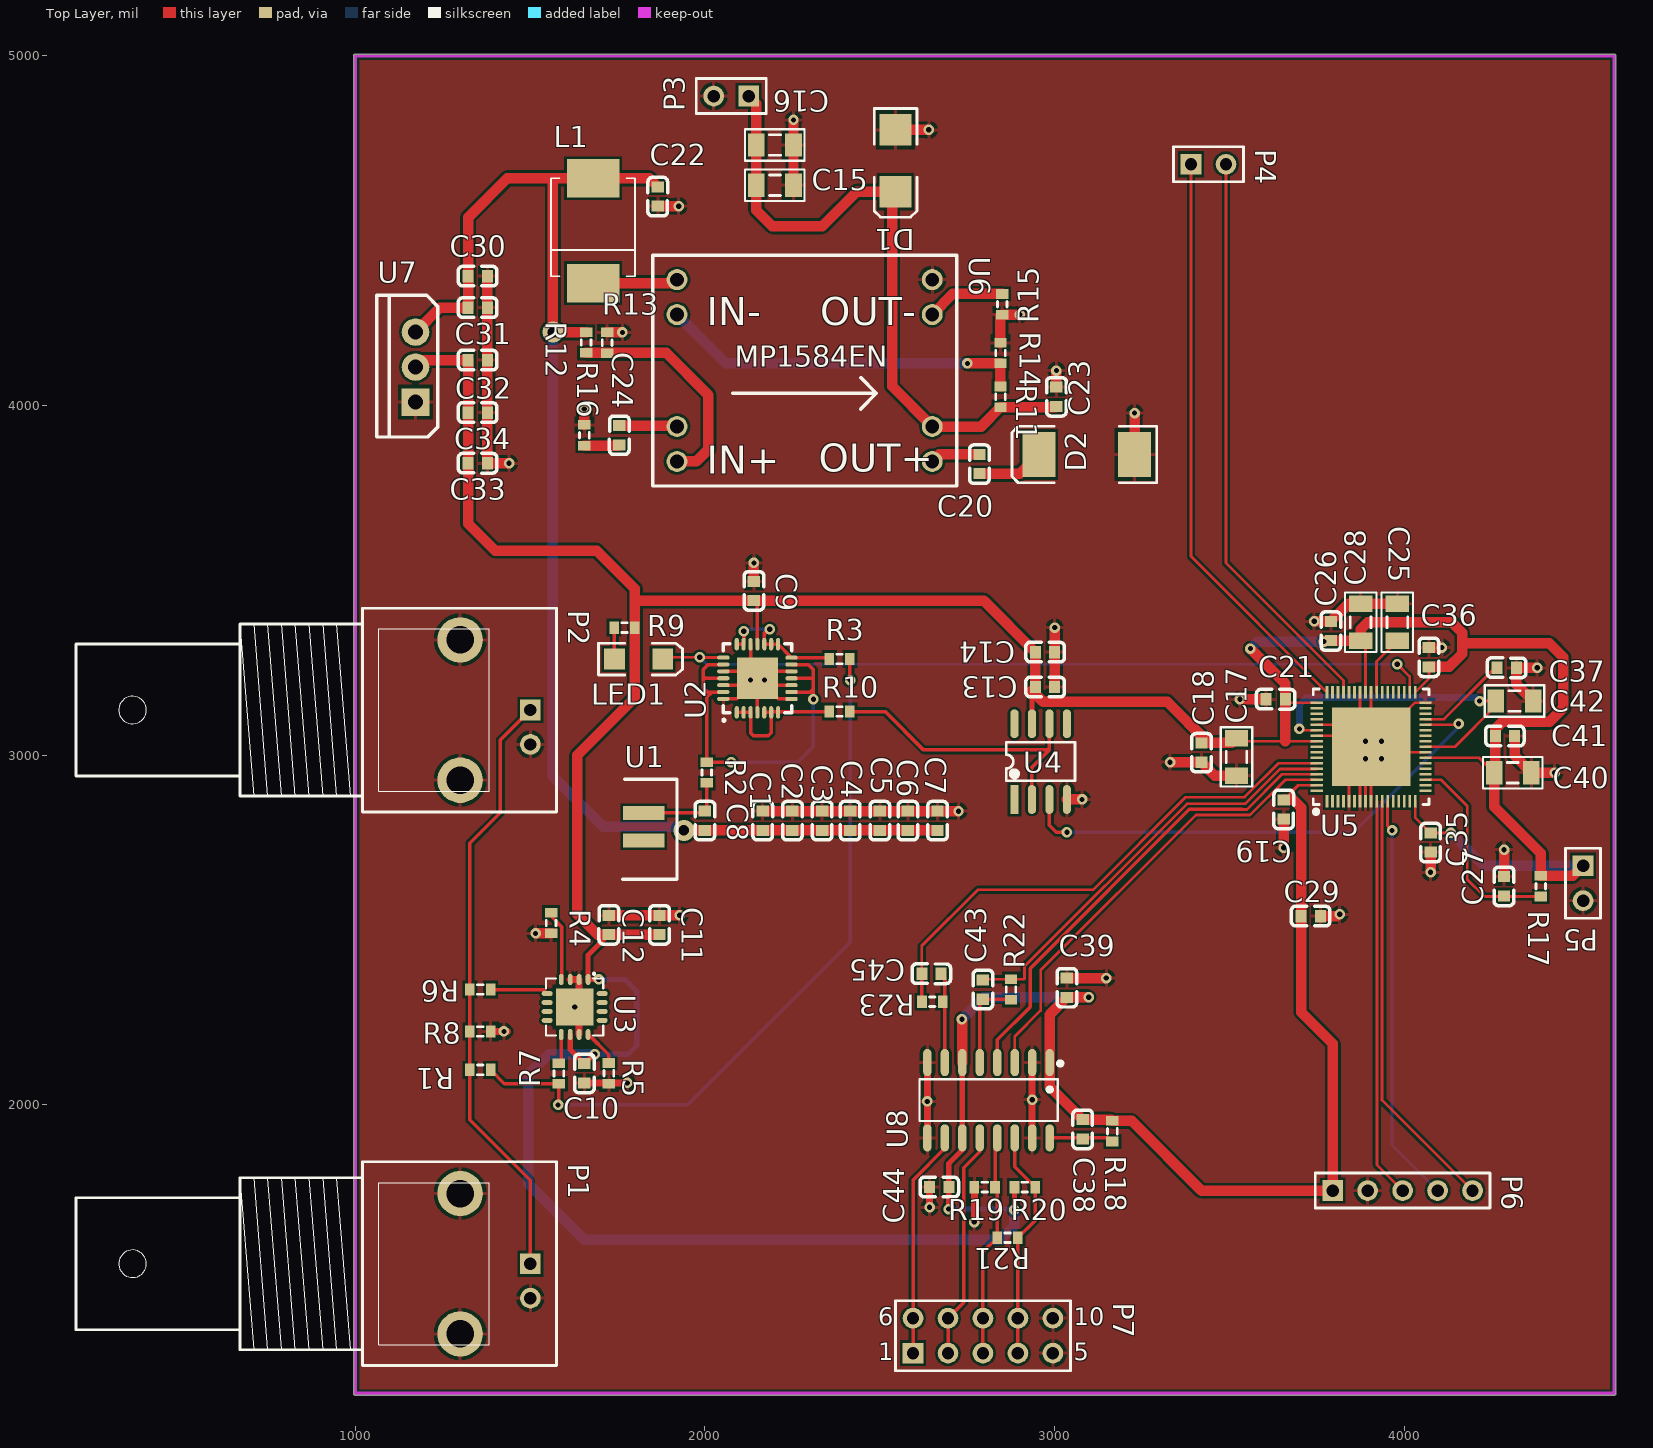
[diagram p0: Top Layer view]
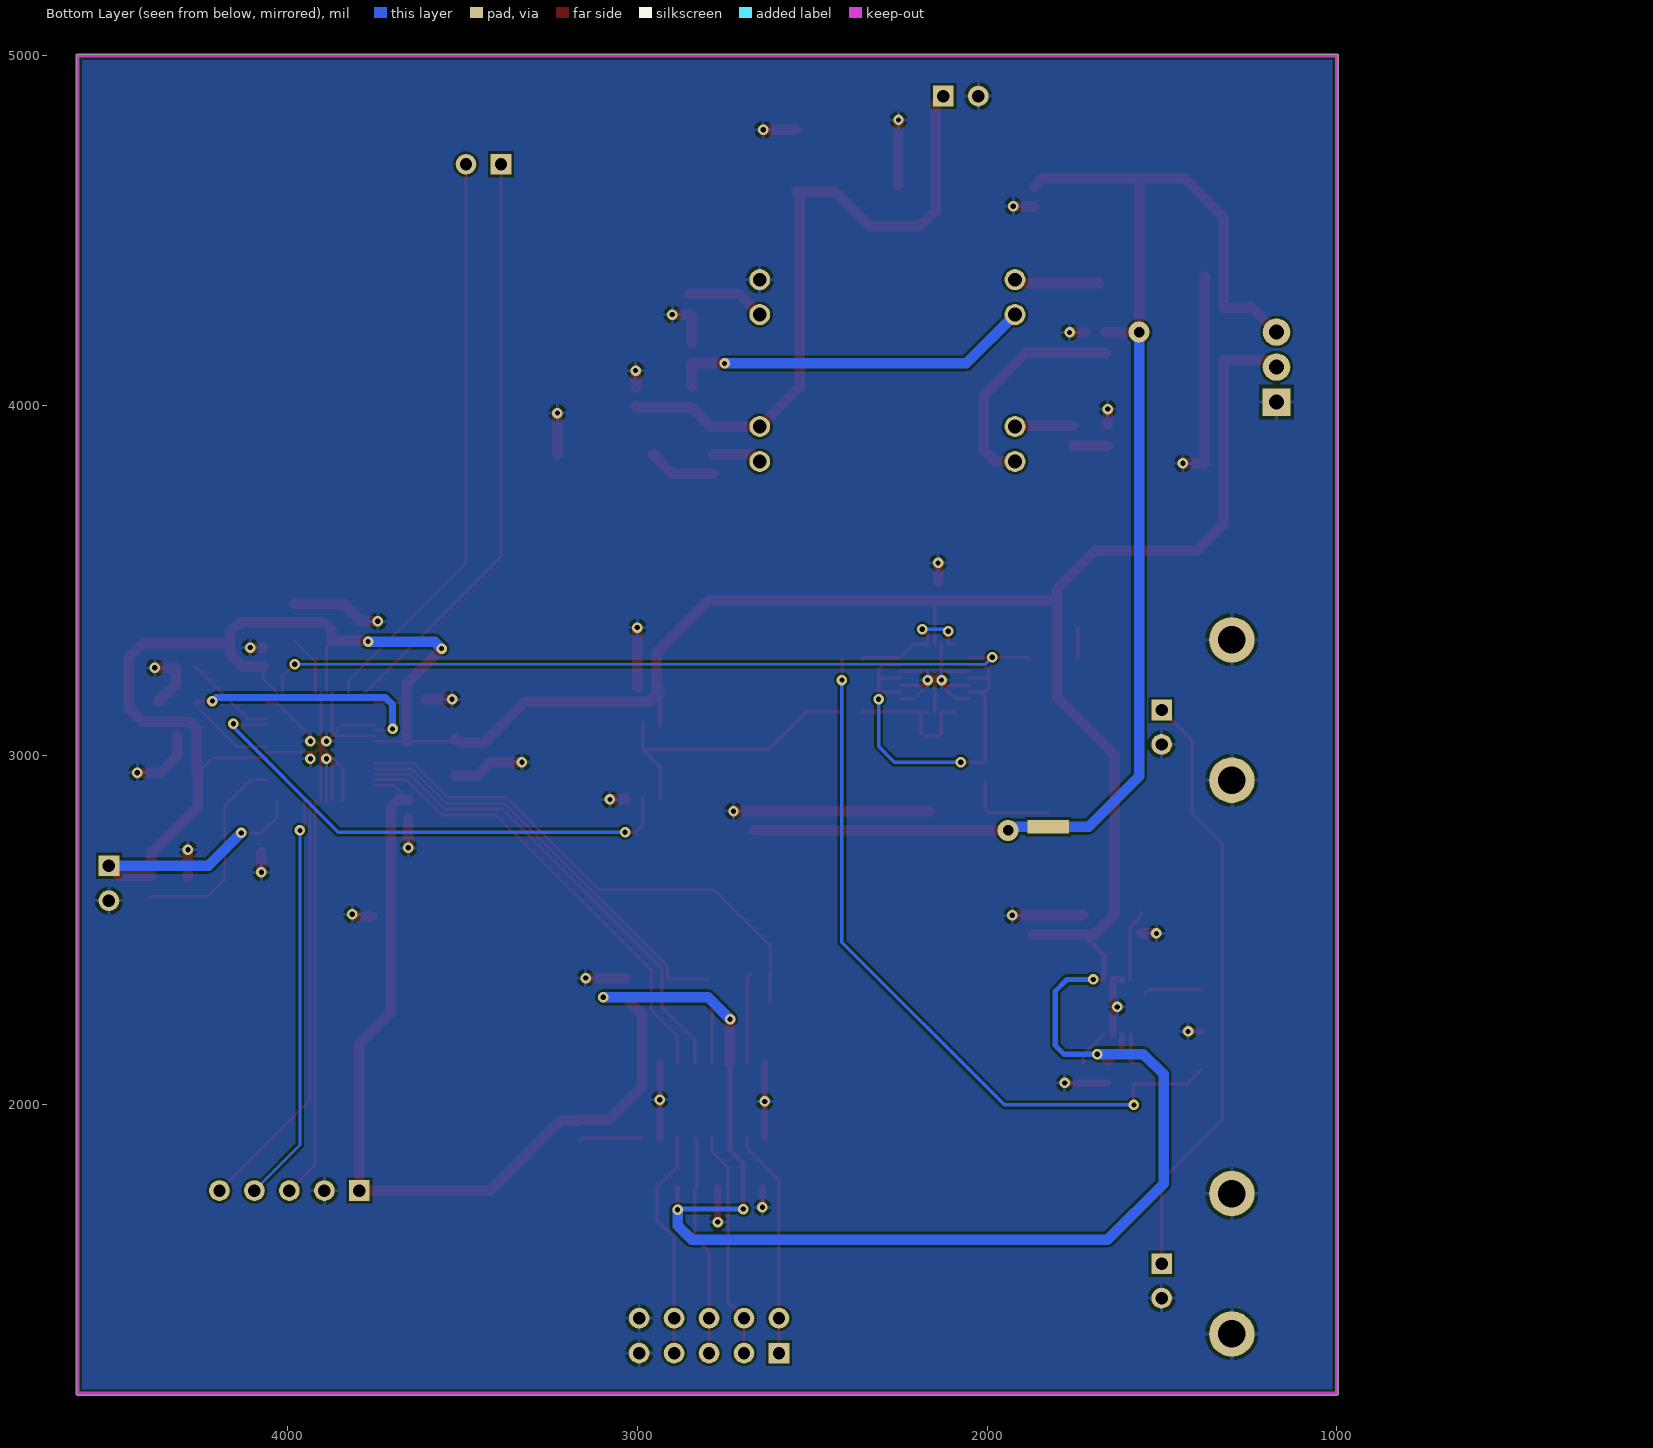
[diagram p1: Bottom Layer view, seen from below]
# Altium PCB MISC80814.PcbDoc
Units mil, origin at the board's own origin, x right, y up, seen from the top; angles counter-clockwise.
Board outline 3610.03 x 3835.03 mil, 2 copper layers (Top Layer, Bottom Layer); 87 components, 46 nets, 326 pads, 64 vias.

## Layer stack, top to bottom (the 12.6 mil dielectric is the usual default, probably not edited)
Top Solder: solder mask 0.4, Solder Resist, Dk 3.5
Top Layer: signal copper 1.4
Dielectric 1: dielectric 12.6, FR-4, Dk 4.8
Bottom Layer: signal copper 1.4
Bottom Solder: solder mask 0.4, Solder Resist, Dk 3.5

## Board outline
1000,1169.98 cw(c1000,1175) 994.99,1175 994.99,5000 cw(c1000,5000) 1000,5005.02 4600,5005.02 cw(c4600,5000) 4605.02,5000 4605.02,1175 cw(c4600,1175) 4600,1169.98

## Design rules (kind name [scope] priority, off if disabled: settings)
Clearance [All] p1: gap=7 except(0: Arc-Text Track-Text SMDPad-Text THPad-Text Via-Text Fill-Text Poly-Text Region-Text Text-Text)
MinimumSolderMaskSliver [All] p1: minsoldermaskwidth=0
PolygonConnect [All] p1: connectstyle=Relief reliefconductorwidth=10 reliefentries=4 polygonreliefangle="90 Angle" airgapwidth=10
RoutingVias [All] p1: holewidth=28 width=50 viastyle="Through Hole" minholewidth=28 minwidth=50 maxholewidth=28 maxwidth=50
SilkToSilkClearance [All] p1: silktosilkclearance=0
SilkToSolderMaskClearance [IsPad] p1: minsilkscreentomaskgap=0 clearancetoexposedcopper=TRUE
SolderMaskExpansion [All] p1: expansion=4
Width [All] p1: maxlimit=30 minlimit=7 preferedwidth=7
27 further rules are at their usual default settings.

## Components (designator, comment, footprint, x,y, rotation, side; value= is the part's Value field where it differs from the comment)
C1 "10UF" C0603 2165.11,2812.75 r270 top
C2 "10UF" C0603 2250.11,2812.75 r270 top
C3 "10UF" C0603 2335.11,2812.75 r270 top
C4 "10UF" C0603 2415.21,2812.75 r270 top
C5 "10UF" C0603 2500.21,2812.75 r270 top
C6 "0.1UF" C0603 2580.11,2812.75 r270 top
C7 "10UF" C0603 2665.21,2812.75 r270 top
C8 "100PF" C0603 2000,2812.75 r270 top
C9 "10UF" C0603 2140,3470 r270 top
C10 "0.1UF" C0603 1655,2090 r90 top
C11 "0.1UF" C0603 1870,2515 r270 top
C12 "10UF" C0603 1725,2515 r270 top
C13 "0.1UF" C0603 2972.86,3194.89 r180 top
C14 "10UF" C0603 2972.86,3294.89 r180 top
C15 "10UF/50V" C1206 2200,4630 r180 top
C16 "10UF/50V" C1206 2200,4745 r180 top
C17 "1UF/16V" C1206 3520,2995 r90 top
C18 "0.1UF" C0603 3419.89,3007.14 r90 top
C19 "0.1UF" C0603 3655,2845 r270 top
C20 "0.1UF" C0603 2784.89,3832.25 r90 top
C21 "0.1UF" C0603 3632.14,3160.11 r0 top
C22 "22UF" C0603 1864.89,4597.25 r90 top
C23 "10UF" C0603 3005,4025 r90 top
C24 "150PF" C0603 1755,3915 r270 top
C25 "1UF/16V" C1206 3980,3380 r270 top
C26 "0.1UF" C0603 3790,3355 r90 top
C27 "10nf" C0603 4285,2625 r90 top
C28 "1UF/16V" C1206 3875,3380 r90 top
C29 "0.1UF" C0603 3732.14,2540.11 r0 top
C30 "10UF" C0603 1350,4370 r0 top
C31 "0.1UF" C0603 1350,4280 r0 top
C32 "10UF" C0603 1350,4130 r0 top
C33 "1UF" C0603 1350,3835 r0 top
C34 "0.1UF" C0603 1350,3980 r0 top
C35 "0.1UF" C0603 4075,2750 r90 top
C36 "0.1UF" C0603 4070,3280 r90 top
C37 "0.1UF" C0603 4292.25,3250.11 r0 top
C38 "12PF" C0603 3080,1930 r90 top
C39 "0.1UF" C0603 3035,2335 r90 top
C40 "1UF/16V" C1206 4310,2950 r0 top
C41 "0.1UF" C0603 4287.25,3055.11 r0 top
C42 "1UF/16V" C1206 4315,3155 r0 top
C43 "12PF" C0603 2795,2330 r270 top
C44 "01.UF" C0603 2670,1765 r180 top
C45 "12PF" C0603 2647.25,2375.11 r0 top
D1 "D Schottky" SMB 2545,4700 r270 top
D2 "S320" SMC 3091.81,3860 r180 top
L1 "22UH" DIODE_SMC 1680,4500 r90 top
LED1 "LED2" 3.2X1.6X1.1 1810,3275 r0 top
P1 "BNC" "BNC_RA CON" 1500.79,1545.79 r0 top
P2 "BNC" "BNC_RA CON" 1500.79,3129.21 r0 top
P3 "Header 2" HDR1X2 2125,4885 r180 top
P4 "Header 2" HDR1X2 3390,4690 r0 top
P5 "Header 2" HDR1X2 4511.06,2683.94 r270 top
P6 "Header 5" HDR1X5 3795,1755 r0 top
P7 "Header 5X2A" HDR2X5_CEN 2595,1290 r0 top
R1 "N/A" J1-0603 1357.36,2100 r180 top
R2 "0.1" J1-0603 2005,2950.47 r270 top
R3 "33" J1-0603 2385,3275 r0 top
R4 "4.7K" J1-0603 1560,2520 r270 top
R5 "4.7K" J1-0603 1725,2090.47 r90 top
R6 "33" J1-0603 1357.36,2330 r180 top
R7 "0" J1-0603 1582.36,2090 r90 top
R8 "510" J1-0603 1357.36,2210 r0 top
R9 "10K" J1-0603 1770,3365 r0 top
R10 "33" J1-0603 2385,3125 r0 top
R11 "100K" J1-0603 2845,4025 r270 top
R12 "300K" J1-0603 1660,4180 r270 top
R13 "39K" J1-0603 1720,4179.53 r90 top
R14 "25K" J1-0603 2845,4150 r270 top
R15 "100K" J1-0603 2850,4289.53 r90 top
R16 "100K" J1-0603 1655,3915 r270 top
R17 "10K" J1-0603 4390,2625.47 r90 top
R18 "820" J1-0603 3165,1925 r270 top
R19 "510" J1-0603 2800,1765 r0 top
R20 "510" J1-0603 2914.53,1765 r0 top
R21 "120" J1-0603 2865,1620 r180 top
R22 "10K" J1-0603 2875,2330 r90 top
R23 "820" J1-0603 2650,2295 r0 top
U1 "Laser diode" 激光二极管 1842.5,2788.13 r90 top
U2 "IC-HG" QFN28-5X5 2150,3216.9 r90 top
U3 "ISL55111IRZ-T" QFN-16_L4.0-W4.0-P0.65-BL-EP2.6 20549.52,-13800.4 r180 top
U4 "OPA335AIDRG4" SOP8 2885,2873.46 r90 top
U5 "CY8C3245LTI-163" QFN-68_L8.0-W8.0-P0.40-TL-EP5.7 3905,3015 r90 top
U6 "MP1584ENZ" MP1548EN 2285,4100 r0 top
U7 "LM317" TO220A 1172.2,4110 r90 top
U8 "IL3122-3E" SOIC-16_L9.9-W3.9-P1.27-LS6.0-BL 2815.9,2013.5 r180 top

## Footprints (in the part's own frame and the unit in brackets; to place one, negate y for a bottom-side part, rotate by r counter-clockwise, add the part's x,y. Pads: shape width x height; smd on the part's side, far side on the other; paste and mask are expansions set on the pad)
3.2X1.6X1.1 [mm] "SMT LED; 2 Flat Leads"
  rect 1.5x1.5 smd: 1(-1.75,0) 2(1.75,0)
  silkscreen extent -2.9,-1.15 3.2,1.15
"BNC_RA CON" [mm] "Connector; BNC Elbow"
  rect 1.5x1.5 hole 0.9: 1(0,0)
  round 3.3 hole 2: 2(-5.1,-5.1) 2(-5.1,5.1)
  round 1.5 hole 0.9: 2(0,-2.5)
  silkscreen extent -33,-7.4 1.9,7.4
C0603 [mm]
  rect 0.8x0.9 smd paste+0 mask+0.051: 1(-0.692,-0.003) 2(0.708,-0.003)
  silkscreen extent -1.4,-0.71 1.4,0.71
C1206 [mm]
  rect 1.2x1.7 smd: 1(-1.35,0) 2(1.35,0)
  silkscreen extent -2.16,-1.14 2.16,1.14, body extent -1.7,-0.9 1.7,0.9, height 1.3
DIODE_SMC [mil] "Diode; 2 Leads"
  rect 110x150 smd: 1(-150,0) 2(150,0)
  silkscreen extent -130,-120 150,120
HDR1X2 [mm] "Connector; Header; 2 Position"
  rect 1.5x1.5 hole 0.9: 1(0,0)
  round 1.5 hole 0.9: 2(2.54,0)
  silkscreen extent -1.27,-1.27 3.81,1.27
HDR1X5 [mm] "Connector; Header; 5 Position"
  rect 1.5x1.5 hole 0.9: 1(0,0)
  round 1.5 hole 0.9: 2(2.54,0) 3(5.08,0) 4(7.62,0) 5(10.16,0)
  silkscreen extent -1.27,-1.27 11.43,1.27
HDR2X5_CEN [mm] "Connector; Header; 5x2 Position"
  rect 1.5x1.5 hole 0.9: 1(0,0)
  round 1.5 hole 0.9: 2(2.54,0) 3(5.08,0) 4(7.62,0) 5(10.16,0) 6(0,2.54) 7(2.54,2.54) 8(5.08,2.54) 9(7.62,2.54) 10(10.16,2.54)
  silkscreen extent -1.27,-1.27 11.43,3.81
J1-0603 [mm] "Chip Resistor, Body 1.6x0.8mm, IPC High Density"
  rect 0.7x0.9 smd: 1(-0.75,0) 2(0.75,0)
  silkscreen extent -0.2,-0.35 0.2,0.35, body extent -0.85,-0.48 0.85,0.48, height 0.9
MP1548EN [mil]
  round 60 hole 39.37 paste+4 mask+4: 1(-365.04,260) 2(-365.04,160) 3(-365.04,-160) 4(-365.04,-260) 5(364.96,260) 6(364.96,160) 7(364.96,-160) 8(364.96,-260)
  silkscreen extent -435,-330 435,330
QFN28-5X5 [mm]
  oval 0.9x0.3 smd paste+0 mask+0.051: 1(-2.397,1.5) 2(-2.397,1) 3(-2.397,0.5) 4(-2.397,0) 5(-2.397,-0.5) 6(-2.397,-1) 7(-2.397,-1.5) 15(2.555,-1.5) 16(2.555,-1) 17(2.555,-0.5) 18(2.555,0) 19(2.555,0.5) 20(2.555,1) 21(2.555,1.5)
  oval 0.3x0.9 smd paste+0 mask+0.051: 8(-1.421,-2.476) 9(-0.921,-2.476) 10(-0.421,-2.476) 11(0.079,-2.476) 12(0.579,-2.476) 13(1.079,-2.476) 14(1.579,-2.476) 22(1.579,2.476) 23(1.079,2.476) 24(0.579,2.476) 25(0.079,2.476) 26(-0.421,2.476) 27(-0.921,2.476) 28(-1.421,2.476)
  rect 3x3 smd paste+0 mask+0.051: 29(0.079,0)
  silkscreen extent -3.01,-2.5 2.58,2.5
QFN-16_L4.0-W4.0-P0.65-BL-EP2.6 [mm]
  oval 0.35x0.8 smd paste-100 mask+0.051: 1(479.648,-410.441) 2(480.298,-410.441) 3(480.948,-410.441) 4(481.598,-410.441) 9(481.598,-406.444) 10(480.948,-406.444) 11(480.298,-406.444) 12(479.648,-406.444)
  oval 0.8x0.35 smd paste-100 mask+0.051: 5(482.621,-409.417) 6(482.621,-408.767) 7(482.621,-408.117) 8(482.621,-407.467) 13(478.624,-407.467) 14(478.624,-408.117) 15(478.624,-408.767) 16(478.624,-409.417)
  rect 2.7x2.7 smd paste-100 mask+0.051: 17(480.623,-408.442)
  silkscreen extent 478.55,-410.93 482.7,-406.37
QFN-68_L8.0-W8.0-P0.40-TL-EP5.7 [mm]
  rect 0.9x0.2 smd paste-100 mask+0.051: 1(-3.713,3.2) 2(-3.713,2.8) 3(-3.713,2.4) 4(-3.713,2) 5(-3.713,1.6) 6(-3.713,1.2) 7(-3.713,0.8) 8(-3.713,0.4) 9(-3.713,0) 10(-3.713,-0.4) 11(-3.713,-0.8) 12(-3.713,-1.2) 13(-3.713,-1.6) 14(-3.713,-2) 15(-3.713,-2.4) 16(-3.713,-2.8) 17(-3.713,-3.2) 35(4.187,-3.2) 36(4.187,-2.8) 37(4.187,-2.4) 38(4.187,-2) 39(4.187,-1.6) 40(4.187,-1.2) 41(4.187,-0.8) 42(4.187,-0.4) 43(4.187,0) 44(4.187,0.4) 45(4.187,0.8) 46(4.187,1.2) 47(4.187,1.6) 48(4.187,2) 49(4.187,2.4) 50(4.187,2.8) 51(4.187,3.2)
  rect 0.2x0.9 smd paste-100 mask+0.051: 18(-2.963,-3.95) 19(-2.563,-3.95) 20(-2.163,-3.95) 21(-1.763,-3.95) 22(-1.363,-3.95) 23(-0.963,-3.95) 24(-0.563,-3.95) 25(-0.163,-3.95) 26(0.237,-3.95) 27(0.637,-3.95) 28(1.037,-3.95) 29(1.437,-3.95) 30(1.837,-3.95) 31(2.237,-3.95) 32(2.637,-3.95) 33(3.037,-3.95) 34(3.437,-3.95) 52(3.437,3.95) 53(3.037,3.95) 54(2.637,3.95) 55(2.237,3.95) 56(1.837,3.95) 57(1.437,3.95) 58(1.037,3.95) 59(0.637,3.95) 60(0.237,3.95) 61(-0.163,3.95) 62(-0.563,3.95) 63(-0.963,3.95) 64(-1.363,3.95) 65(-1.763,3.95) 66(-2.163,3.95) 67(-2.563,3.95) 68(-2.963,3.95)
  rect 5.7x5.7 smd paste-100 mask+0.051: 69(0.237,0)
  silkscreen extent -4.64,-4.2 4.44,4.2
SMB [mm] "DO-214-AA/SMB; 2 C-Bend Leads; Body 5.3 x 3.6 mm, inc. leads (LxW)"
  rect 2.3x2.3 smd: 1(-2.25,0) 2(2.25,0)
  silkscreen extent -3.8,-1.55 4.1,1.55
SMC [mm] "DO-214-AB/SMC; 2 C-Bend Leads; Body 7.9 x 5.9 mm, inc. leads (LxW)"
  rect 2.4x3.3 smd: 1(-3.475,0) 2(3.475,0)
  silkscreen extent -5.07,-2.05 5.43,2.05
SOIC-16_L9.9-W3.9-P1.27-LS6.0-BL [mil]
  oval 23.7x77.6 smd paste+0 mask+2: 1(-169.99,-107.7) 2(-119.99,-107.7) 3(-69.99,-107.7) 4(-19.99,-107.7) 5(30.01,-107.7) 6(80.01,-107.7) 7(130.01,-107.7) 8(180.01,-107.7) 9(180.01,107.7) 10(130.01,107.7) 11(80.01,107.7) 12(30.01,107.7) 13(-19.99,107.7) 14(-69.99,107.7) 15(-119.99,107.7) 16(-169.99,107.7)
  silkscreen extent -206,-111 203,60
SOP8 [mm]
  rect 2.1x0.6 smd: 1(0,0)
  oval 2.1x0.6 smd: 2(0,-1.27) 3(0,-2.54) 4(0,-3.81) 5(5.5,-3.81) 6(5.5,-2.54) 7(5.5,-1.27) 8(5.5,0)
  silkscreen extent 1.35,-4.41 4.15,0.6, body extent -0.21,-4.4 5.8,0.6, height 1.9
TO220A [mm] "220，3脚晶体管"
  rect 2x2 hole 1.1: 1(-2.54,0)
  round 2 hole 1.1: 2(0,0) 3(2.54,0)
  silkscreen extent -5.08,-1.6 5.21,2.82, body extent -5.08,-1.45 5.22,2.98, height 18.5
激光二极管 [mm]
  rect 1x3 smd paste+0 mask+0.051: 1(1.19,0.445) 3(-0.809,0.444)
  rect 1x3 smd far side paste+0 mask+0.051: 2(0.19,0.445)
  silkscreen extent -3.62,-1.97 3.62,1.97

## Part data
C1 C2 C3 C4 C5 C6 C7 C8 C9 C10 C11 C12 C13 C14 C15 C16 C17 C18 C19 C20 C21 C22 C23 C24 C25 C26 C27 C28 C29 C30 C31 C32 C33 C34 C35 C36 C37 C38 C39 C40 C41 C42 C43 C44 C45: library part "Cap Semi", "Capacitor (Semiconductor SIM Model)"
D1: "Schottky Diode"
D2: library part Diode, "Default Diode"
L1: library part "Inductor Iron Dot", "Magnetic-Core Inductor with Winding Polarity Marking"
LED1: "Typical RED, GREEN, YELLOW, AMBER GaAs LED"
P1 P2: "BNC Elbow Connector"
P3 P4 P5: "Header, 2-Pin"
P6: "Header, 5-Pin"
P7: "Header, 5-Pin, Dual row"
R1 R2 R3 R4 R5 R6 R7 R8 R9 R10 R11 R12 R13 R14 R15 R16 R17 R18 R19 R20 R21 R22 R23: library part Res2, "Resistor"
U1: library part 激光二极管
U6: library part MP1584ENZ_own
U7: "Adjustable linear regulator IC"

## Via types
v1: diameter 30, hole 15, Top Layer to Bottom Layer, 62 vias
v2: diameter 60, hole 30, Top Layer to Bottom Layer, 2 vias

## Nets (pads, with @x,y where several pads share a name; then routed paths per layer and width w, separated by ;. In a path a pad name is that pad's centre, name@x,y a point inside that pad or via, vN(x,y) a via of type N, cw(c..) or ccw(c..) an arc to the next point about the centre after c; other vN are vias at no path point)
A: P7.4 P7.9 R20.2 R21.1 U8.14 | length 660.6
  Top Layer w10: U8.14 2885.88,1823.17 R20.2 2944.06,1669.53 R21.1 2895,1619.53 P7.9 P7.4
B: P7.3 P7.8 R19.2 R21.2 U8.13 | length 637.7
  Top Layer w10: P7.3 P7.8 2795,1579.53 R21.2 2835.47,1759.06 R19.2 2829.53,1899.44 U8.13
CL_V: R10.2 U4.2 U4.6 | length 853.3
  Top Layer w10: R10.2 2515,3125 2625,3015 2985,3015 ; U4.2 2935,2965 2985,3015 ; U4.6 2985,3015
DAC_OUT: U4.3 U5.30 | length 1481.6
  Top Layer w8: U5.30 4152.33,3087.33 v1(4155,3090)
  Top Layer w10: U4.3 2985,2800 3005,2780 v1(3035,2780)
  Bottom Layer w10: v1(3035,2780) 3855,2780 4155,3080 v1(4155,3090)
DE: C43.1 R22.2 U5.64 | length 1225.5
  Top Layer w8: C43.1 2797.18,2359.53 R22.2 2912.15,2359.53 2914,2361.37 2914,2396.63 3378.37,2861 3544.79,2861 3644.38,2960.59 3748.74,2960.59 U5.64
EN_IN: R1.1 R3.2 R7.1 | length 2111.1
  Top Layer w10: R1.1 1426.42,2060.47 R7.1 1582.36,2002.36 v1(1580,2000) ; R3.2 2414.53,3215.47 v1(2415,3215)
  Bottom Layer w10: v1(1580,2000) 1950,2000 2415,2465 v1(2415,3215)
EORR: LED1.2 U2.22 U5.36 | length 2274.1
  Top Layer w8: LED1.2 1883.9,3280 v1(1985,3280) 1985.94,3279.06 U2.22 ; v1(3980,3260) 4015.24,3224.76 U5.36
  Bottom Layer w8: v1(1985,3280) 2005,3260 v1(3980,3260)
GND: C1.1 C2.1 C3.1 C4.1 C5.1 C6.1 C7.1 C9.1 C10.1 C11.1 C12.1 C13.1 C14.1 C15.1 C16.1 C17.1 C18.1 C19.2 C21.1 C22.1 C23.2 C25.1 C26.2 C27.2 C28.2 C29.2 C30.2 C31.2 C32.2 C33.2 C34.2 C35.1 C36.2 C37.2 C39.2 C40.2 C41.2 C42.2 C44.2 D1.1 D2.1 P1.2 P2.2 P3.2 P5.2 P6.2 P7.5 P7.10 R4.2 R5.1 R8.2 R13.2 R14.1 R15.1 R16.1 R19.1 U2.4 U2.8 U2.10 U2.12 U2.19 U2.24 U2.26 U2.28 U2.29 U3.2 U3.3 U3.11 U3.17 U4.4 U5.5 U5.7 U5.8 U5.9 U5.25 U5.34 U5.43 U5.45 U5.56 U5.58 U5.69 U6.5 U7.1 U8.2 U8.8 U8.9 U8.15 | length 7009.8
  Top Layer w8: U5.58 3873.5,3055.83 3842,3087.33 U5.56 ; U5.5 3842.01,2961.34 U5.69@3873.51,2992.84 ; U5.7 U5.69@3873.51,2992.84 ; U5.45 3873.51,3055.82 U5.69 ; U5.8 U5.69@3889.25,3008.58 ; U5.9 U5.69 ; U5.43 U5.69 ; U5.25 3920.74,3008.59 U5.69 ; U5.34 4030.99,3150.32 U5.69 ; U5.69@3873.51,2992.84 U5.69@3889.25,3008.58 ; U5.69@3889.25,3008.58 U5.69
  Top Layer w10: U2.28 2090.94,3160.94 U2.29@2125,3195 ; U2.26 2119.68,3200.32 U2.29@2125,3195 ; U2.24 U2.29@2130.31,3239.69 ; U2.19 U2.29@2130.32,3239.68 ; U2.4 U2.29 ; U2.8 2209.06,3160.94 U2.29@2169.68,3200.32 ; U2.10 U2.29@2169.68,3200.32 ; U2.12 2169.69,3239.69 U2.29 ; U2.29@2125,3195 U2.29 ; U2.29@2130.32,3239.68 U2.29 ; U2.29 U2.29@2169.68,3200.32
  Top Layer w20: R8.2 v1@1435,2210 ; U3.3 U3.2 1640.16,2292.8 v1(1627.36,2280) 1640.16,2267.2 U3.11 ; C10.1 v1(1777.75,2062.75) ; U8.9 U8.8 ; v1(2642.14,1707.14) C44.2 ; v1@2770.47,1664.53 R19.1 ; U8.15 U8.2
  Top Layer w30: C30.2 C31.2 C32.2 C34.2 C33.2 v1(1439.89,3834.89) ; v1(1515.47,2490.47) R4.2 ; R16.1 v1(1655,3990) ; R13.2 v1(1764.06,4209.06) ; C12.1 C11.1 v1(1927.75,2542.25) ; C22.1 v1(1925,4570) ; C9.1 v1(2139.89,3549.89) ; C1.1 C2.1 C3.1 C4.1 C5.1 C6.1 C7.1 v1(2725,2840) ; C15.1 C16.1 v1(2253.15,4816.85) ; D1.1 v1(2640,4788.58) ; R14.1 2845,4255 R15.1 v1(2900,4260) ; C13.1 C14.1 v1(3000.11,3365.11) ; C23.2 v1@3005.11,4099.89 ; U4.4 v1(3078.46,2873.46) ; C39.2 v1(3147.86,2362.86) ; D2.1 v1(3228.62,3978.62) ; v1(3330.11,2979.89) C18.1 3458.04,2941.85 C17.1 ; v1(3530,3160) C21.1 ; v1(3654.89,2735.11) C19.2 ; v1(3742.14,3382.86) C26.2 3840.39,3433.15 C28.2 C25.1 ; C29.2 v1@3805,2540 ; C36.2 v1(4107.14,3307.86) ; v1(4075.11,2665.11) C35.1 ; C27.2 v1(4285.11,2729.89) ; C41.2 4315.11,2998.04 C40.2 v1(4430,2950) ; C42.2 4320.11,3203.04 C37.2 v1(4380,3250)
  other v1: 2770,1665 2635.88,2010 2935.88,2015 1425,2210 3815,2545 3889.25,2990 3935,2990 3889.26,3040.08 3935,3040 2130,3215 2170,3215 3005,4100
NetC8_1: C8.1 R2.2 U1.1 | length 260
  Top Layer w10: U1.1 1994.89,2835 C8.1 2005,2845.11 R2.2
NetC20_1: C20.1 D2.2 | length 192.8
  Top Layer w30: C20.1 2900,3805 D2.2
NetC20_2: C20.2 U6.8 | length 143.4
  Top Layer w30: U6.8 2670.07,3860.11 C20.2
NetC24_1: C24.1 U6.3 | length 166
  Top Layer w30: C24.1 1917.71,3942.25 U6.3
NetC24_2: C24.2 R16.2 | length 100.6
  Top Layer w30: R16.2 1753.23,3885.47 C24.2
NetC25_2: C25.2 U5.42 | length 171.5
  Top Layer w8: U5.42 3920.75,3267.6 C25.2
NetC37_1: C37.1 U5.31 | length 265.3
  Top Layer w8: U5.31 4113.07,3103.07 4260,3250 C37.1
NetC38_1: C38.1 R18.2 U8.16 | length 183.4
  Top Layer w10: U8.16 3154.67,1905.8 R18.2
NetC43_2: C43.2 R22.1 U8.5 | length 265.5
  Top Layer w10: U8.5 2785.88,2293.12 C43.2 2873.34,2302.14 R22.1
NetC45_2: C45.2 R23.2 U8.7 | length 258.3
  Top Layer w10: C45.2 2685.88,2364.23 U8.7
NetL1_1: L1.1 U6.1 | length 244.1
  Top Layer w30: L1.1 1909.96,4350 U6.1
NetLED1_1: LED1.1 R9.1 | length 90.3
  Top Layer w10: R9.1 1741.1,3364.37 LED1.1
NetP1_1: P1.1 P2.1 R1.2 R6.2 R8.1 | length 1726.7
  Top Layer w10: P1.1 1500.79,1784.21 1327.83,1957.17 R1.2 R6.2 1327.83,2747.83 1415,2835 1415,3043.43 P2.1
NetP4_1: P4.1 U5.51 | length 1671.3
  Top Layer w8: P4.1 3390,3568.87 U5.51
NetP4_2: P4.2 U5.48 | length 1649.4
  Top Layer w8: P4.2 3490,3550 3826.26,3213.74 U5.48
NetP6_3: P6.3 U5.10 | length 1144.6
  Top Layer w8: U5.10 3921.5,2868.07 3921.5,1828.5 P6.3
NetP6_4: P6.4 U5.12 | length 1173
  Top Layer w8: U5.12 3952.25,2797.75 v1(3965,2785)
  Bottom Layer w8: v1(3965,2785) 3965,1885 P6.4
NetP6_5: P6.5 U5.11 | length 1220.9
  Top Layer w8: U5.11 3936.5,2013.5 P6.5
NetR2_1: R2.1 U2.9 U2.11 U2.13 U2.23 U2.25 U2.27 | length 1188.6
  Top Layer w10: U2.27 2020,3180.63 ; U2.25 2000,3220 1995,3225 ; U2.23 2009.37,3259.37 1995,3245 1995,3225 ; v1(2075,2980) R2.1 2005,3165.63 2020,3180.63 ; U2.9 2300.63,3180.63 2310,3190 ; U2.11 2305,3220 2310,3225 ; U2.13 2295.63,3259.37 2310,3245 2310,3225 ; v1(2310,3160) 2310,3190 ; 1995,3225 1995,3191.26 2005.63,3180.63 2020,3180.63 ; 2310,3190 2310,3225
  Bottom Layer w10: v1(2075,2980) 2265,2980 2310,3025 v1(2310,3160)
NetR3_1: R3.1 U2.14 U2.15 U2.16 U2.17 U2.20 U2.21 | length 388.4
  Top Layer w10: U2.21 U2.20 v1(2110.63,3354.37) ; v1(2185,3360) 2174.69,3349.69 2169.69,3349.69 U2.17 U2.16 U2.15 U2.14 2351.41,3279.06 R3.1
  Bottom Layer w10: v1(2110.63,3354.37) 2116.26,3360 v1(2185,3360)
NetR4_1: R4.1 U3.4 | length 203.5
  Top Layer w10: R4.1 1560,2539.68 1589.72,2509.96 1589.72,2359.42 U3.4
NetR5_2: R5.2 U3.12 | length 106.5
  Top Layer w10: U3.12 1666.86,2201.32 1725,2143.18 R5.2
NetR6_1: R6.1 U3.5 | length 166.6
  Top Layer w10: R6.1 1537.07,2330 U3.5
NetR7_2: R7.2 U3.9 | length 84.5
  Top Layer w10: R7.2 1588.98,2126.14 U3.9
NetR10_1: R10.1 U2.1 U2.2 U2.3 U2.5 U2.6 U2.7 | length 409.5
  Top Layer w10: U2.1 U2.2 U2.3 2130.32,3064.68 2140,3055 2180,3055 2189.37,3064.37 U2.6 ; U2.5@2170,3122.2 U2.5 U2.6 ; R10.1 2191.86,3125 U2.6
NetR11_1: R11.1 R14.2 U6.2 | length 1048.8
  Top Layer w30: v1(2750.47,4120.47) R14.2 R11.1
  Bottom Layer w30: U6.2 2059.49,4120.47 v1(2750.47,4120.47)
NetR12_2: R12.2 R13.1 U6.4 | length 659.4
  Top Layer w30: R12.2 1889.53,4150.47 2010,4030 2010,3875 1975,3840 U6.4
NetR15_2: R15.2 U6.6 | length 224.5
  Top Layer w30: U6.6 2709.02,4319.06 R15.2
R1: C27.1 R17.1 U5.20 | length 590.8
  Top Layer w8: U5.20 4105.15,2929.85 4180,2855 4180,2645 4229.06,2595.94 R17.1
RE: U5.65 U8.4 | length 1357.4
  Top Layer w8: 3535,2845 3550,2845 3650.59,2945.59 U5.65
  Top Layer w10: U8.4 2835.88,2185.88 2930,2280 2930,2390 3385,2845 3535,2845
RX: U5.66 U8.3 | length 1309.7
  Top Layer w8: U8.3 2885.88,2195.88 2960,2270 2960,2385 3404,2829 3559,2829 3659.85,2929.85 U5.66
TX: C45.1 R23.1 U5.63 | length 1505.9
  Top Layer w8: C45.1 2620,2455 2780,2615 3110,2615 3375,2880 3542.57,2880 3639.67,2977.09 U5.63
  Top Layer w10: C45.1 2620.47,2374.53 R23.1
VCCD: C42.1 U5.26 U5.57 | length 958.3
  Top Layer w8: v1(3700,3075) 3703.42,3071.58 U5.57 ; U5.26 4144.33,3024.33 4261.85,3141.85 C42.1 v1(4215,3155)
  Bottom Layer w20: v1(3700,3075) 3700,3145 3720,3165 4205,3165 v1(4215,3155)
VDD5V: C9.2 C10.2 C11.2 C12.2 C13.2 C14.2 C17.2 C18.2 C19.1 C21.2 C26.1 C28.1 C29.1 C32.1 C33.1 C34.1 C35.2 C36.1 C38.2 C39.1 C40.1 C41.1 C44.1 P5.1 P6.1 R9.2 R17.2 R18.1 R20.1 U2.18 U3.1 U3.10 U4.7 U5.17 U5.24 U5.35 U5.44 U5.52 U5.59 U5.67 U7.2 U8.1 U8.6 U8.11 | length 14984
  Top Layer w8: C17.2 3528.07,3040.08 3660,3040.08 U5.59 ; C19.1 3696.75,2914.1 U5.67 ; C21.2 3669.68,3150.32 U5.52 ; C28.1 3889.25,3312.6 U5.44 ; U5.17 4030.99,2821.98 C35.2 v1(4132.86,2777.86) ; U5.35 4070.11,3218.97 C36.1 ; U5.24 4214.01,2992.84 C40.1
  Top Layer w10: C9.2 2150,3432.03 U2.18
  Top Layer w15: U3.10 1614.57,2158.4 C10.2 1682.24,2145 v1(1685,2145) ; v1(1696.32,2358.68) U3.1 1665.75,2427.99 C12.2 ; v1(2697.25,1702.25) C44.1 2697.25,1832.25 2735.88,1870.88 U8.11 U8.6 ; v1(2885,1700) R20.1 ; U4.7 2935,3185 C13.2
  Top Layer w30: U7.2 1192.1,4129.89 C32.1 C34.1 C33.1 1322.75,3662.25 1400,3585 1690,3585 1799.53,3475.47 1799.53,3450 ; C11.2 C12.2 1692.86,2487.14 1635,2545 1635,3000 1799.53,3164.53 R9.2 1799.53,3450 ; v1(2735,2245) 2735.88,2244.12 U8.6 ; C13.2@2935,3185 2966.66,3153.34 3321.66,3153.34 3440,3035 3506.85,3035 C17.2 ; C13.2 C14.2 2797.86,3442.14 C9.2 1807.39,3442.14 1799.53,3450 ; v1(3097.75,2307.75) C39.1 2985.88,2258.53 U8.1 2985.88,2052.09 C38.2 3161.66,1957.86 R18.1 3220.47,1954.53 3420,1755 P6.1 3795,2175 3704.89,2265.11 C29.1 3704.89,2850.11 3682.75,2872.25 C19.1 ; v1(3560,3305) 3660,3205 C21.2 3660,3040.08 ; v1(3770,3325) 3772.75,3327.75 C26.1 3874.1,3327.75 C28.1 3875,3360 3895,3380 4135,3380 4165,3350 4165,3320 ; C36.1 4127.75,3252.75 4165,3290 4165,3320 ; P5.1 4482.13,2655 R17.2 4390,2720 4256.85,2853.15 C40.1 4260,2953.15 C41.1 4260,3075 4280,3095 4415,3095 4455,3135 4455,3280 4415,3320 4165,3320
  Bottom Layer w15: v1(1685,2145) 1780,2145 1805,2170 1805,2325 1771.32,2358.68 v1(1696.32,2358.68) ; v1(2697.25,1702.25) 2882.75,1702.25 v1(2885,1700)
  Bottom Layer w30: v1(1685,2145) 1552.67,2145 1495,2087.33 1495,1775 1655,1615 2845,1615 2885,1655 v1(2885,1700) ; v1(2735,2245) 2797.75,2307.75 v1(3097.75,2307.75) ; v1(3560,3305) 3580,3325 v1(3770,3325) ; v1(4132.86,2777.86) 4226.79,2683.94 P5.1
VDD8V: C1.2 C2.2 C3.2 C4.2 C5.2 C6.2 C7.2 C8.2 C22.2 C30.1 C31.1 L1.2 R12.1 U1.2 U7.3 | length 4006
  Top Layer w30: U7.3 1242.1,4279.89 C31.1 C30.1 1322.75,4537.75 1435,4650 1565,4650 ; R12.1 1565.47,4209.53 v2(1565,4210) 1565,4650 ; C22.2 1840.11,4650 L1.2 1565,4650 ; v2(1940,2785) 1940.11,2784.89 C8.2 C1.2 C2.2 C3.2 C4.2 C5.2 C6.2 C7.2
  Bottom Layer w30: v2(1565,4210) 1565,2940 1709.37,2795.63 U1.2 1929.37,2795.63 v2(1940,2785)
VDD12V: C15.2 C16.2 C23.1 D1.2 P3.1 R11.2 U6.7 | length 1895.9
  Top Layer w30: P3.1 2146.85,4863.15 C16.2 C15.2 2146.85,4558.15 2192.17,4512.83 2335,4512.83 2433.58,4611.42 D1.2 2535,4601.42 2535,4054.96 U6.7 2789.53,3940 R11.2 3002.82,3995.47 C23.1
Y: P7.1 P7.6 U8.10 | length 653.4
  Top Layer w10: P7.1 P7.6 2595,1785 2685.88,1875.88 U8.10
Z: P7.2 P7.7 U8.12 | length 653.4
  Top Layer w10: P7.2 P7.7 2740,1435 2740,1820 2785.88,1865.88 U8.12
pads on no net: U1.3 U3.6 U3.7 U3.8 U3.13 U3.14 U3.15 U3.16 U4.1 U4.5 U4.8 U5.1 U5.2 U5.3 U5.4 U5.6 U5.13 U5.14 U5.15 U5.16 U5.18 U5.19 U5.21 U5.22 U5.23 U5.27 U5.28 U5.29 U5.32 U5.33 U5.37 U5.38 U5.39 U5.40 U5.41 U5.46 U5.47 U5.49 U5.50 U5.53 U5.54 U5.55 U5.60 U5.61 U5.62 U5.68

## Polygon pours and split planes (outlines as drawn)
GND on Bottom Layer "G" (solid, remove dead copper, pour order 4): 710,5315 745,5350 5105,5350 5105,1165 4675,735 4465,945 405,945
GND on Top Layer "G" (solid, remove dead copper, pour order 6): 440,5400 5125,5400 5175,5350 4685,4860 4685,1000 630,1000 445,815

## Keep-outs
Keep-Out Layer:
  lines w10: 4465,1175 4600,1175 4600,2750 4600,5000 1000,5000 1000,1175 4475,1175